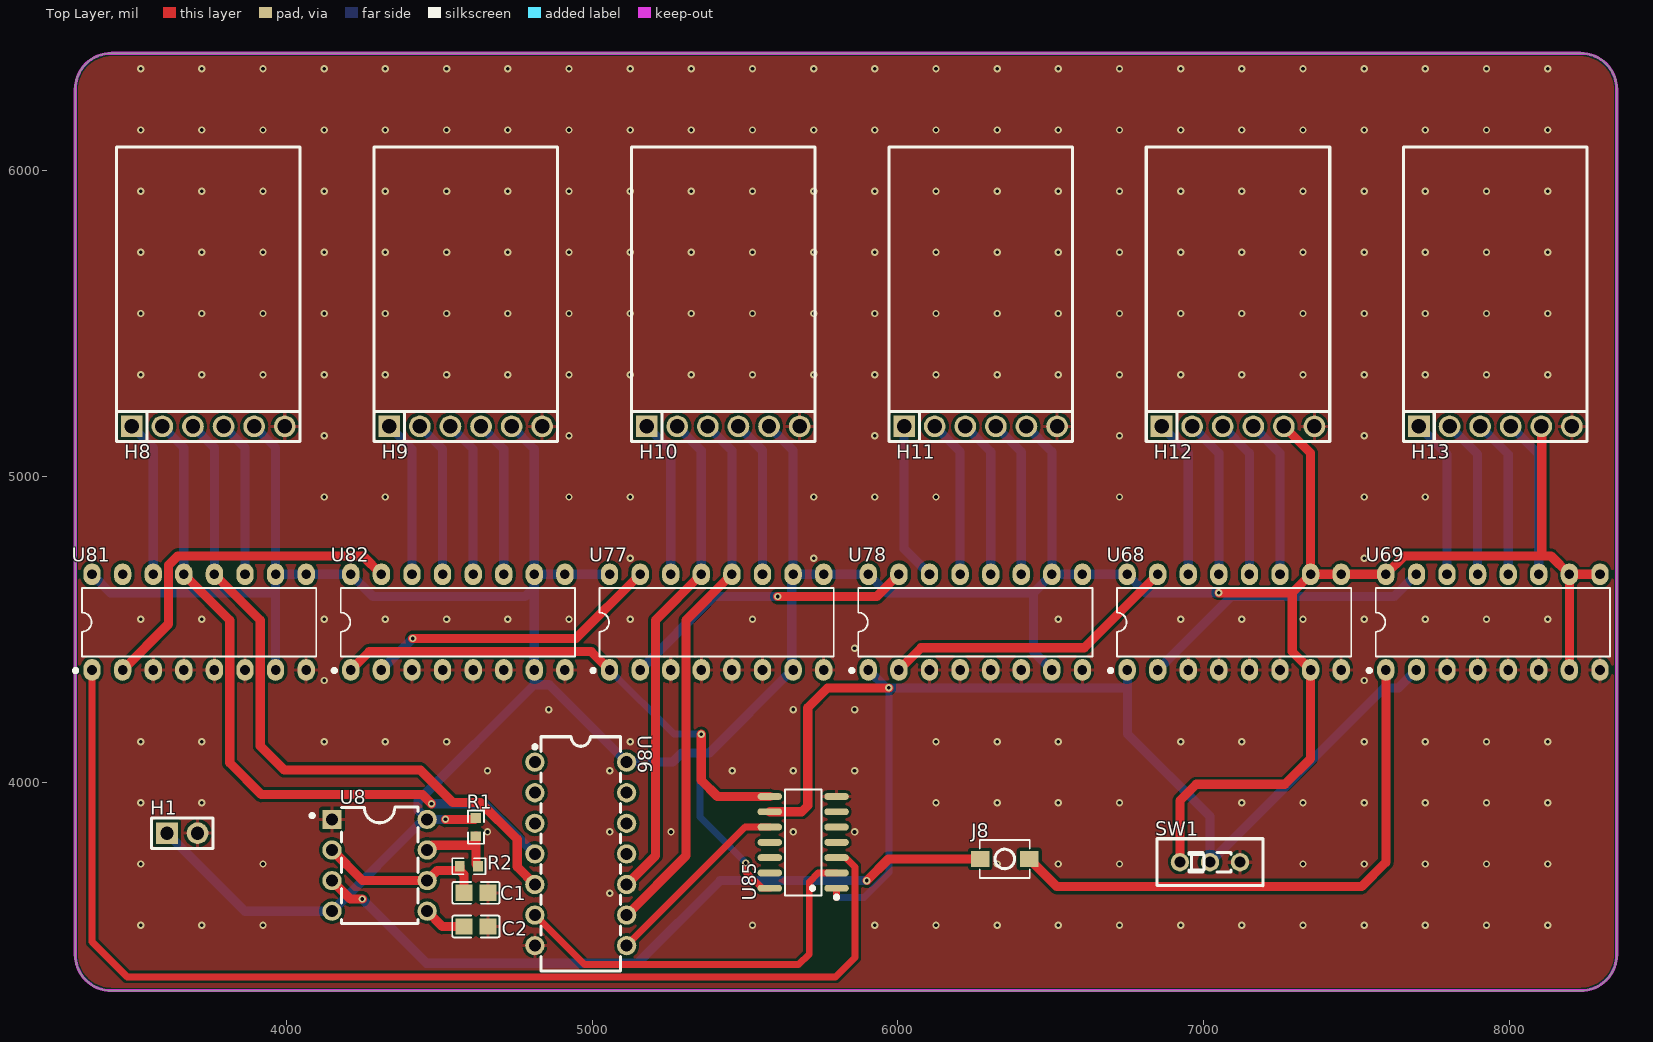
[diagram p0: Top Layer view]
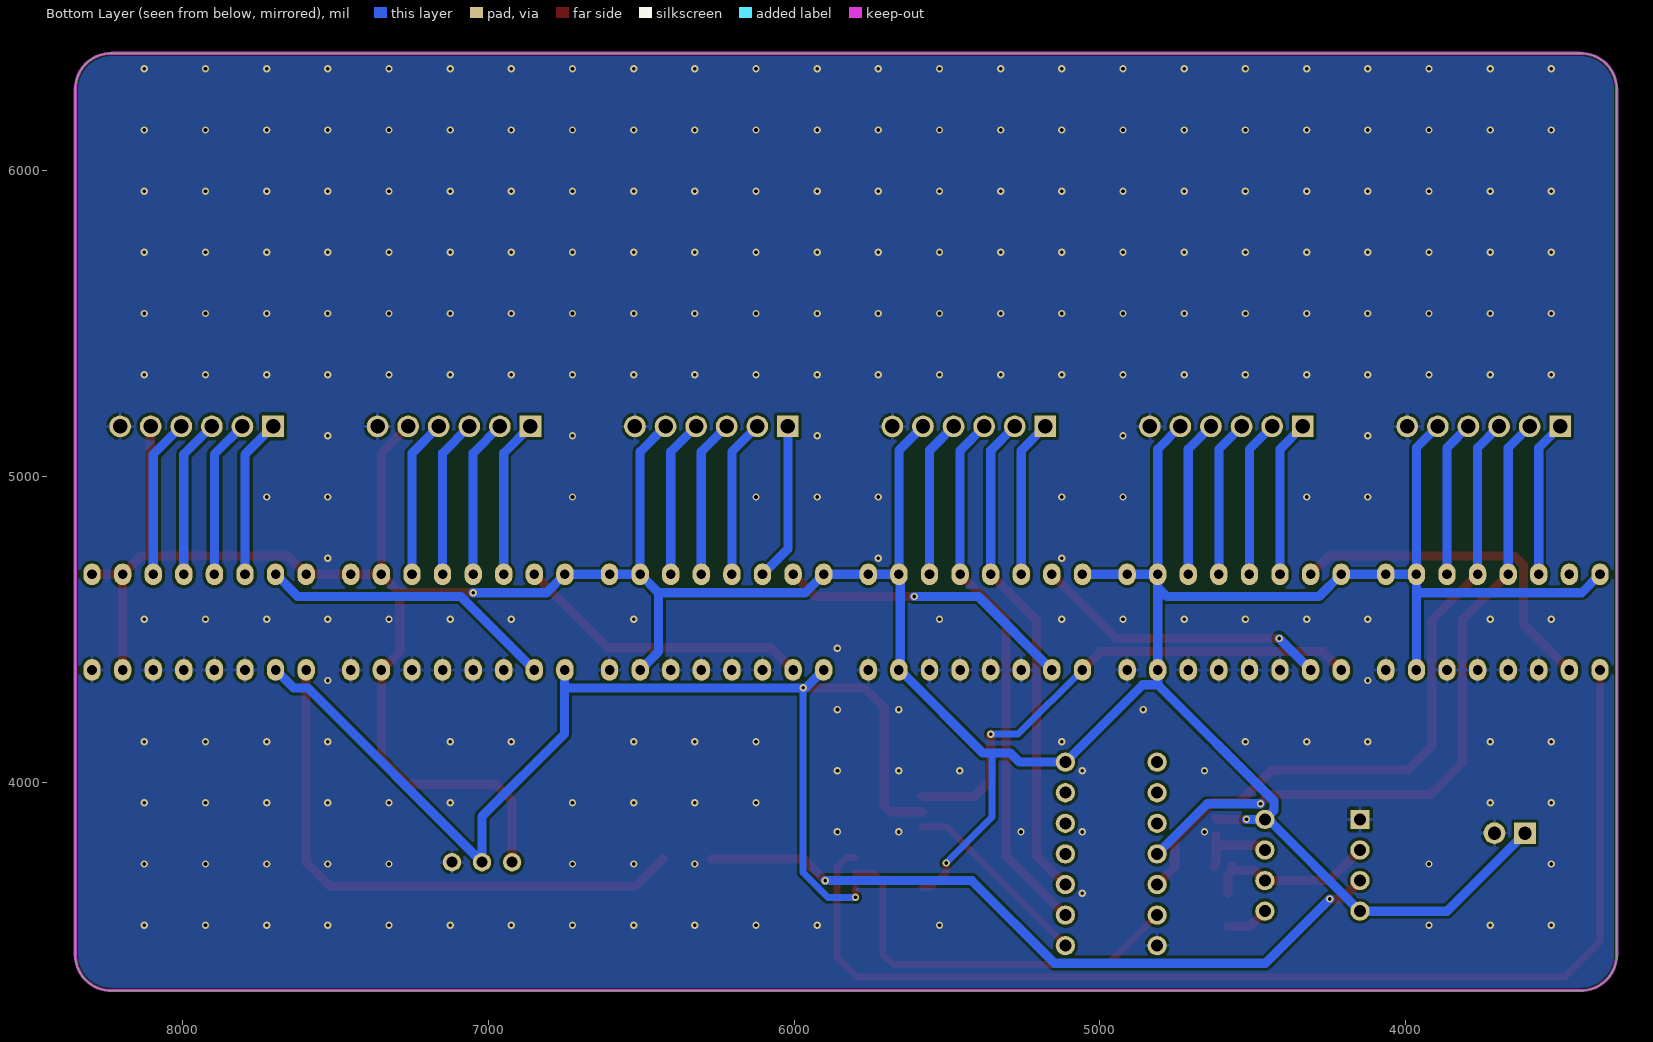
[diagram p1: Bottom Layer view, seen from below]
# Altium PCB MISC51760.pcbdoc
Units mil, origin at the board's own origin, x right, y up, seen from the top; angles counter-clockwise.
Board outline 5040 x 3065 mil, 2 copper layers (Top Layer, Bottom Layer), stack 62.206 mil thick; 22 components, 41 nets, 183 pads, 260 vias.

## Layer stack, top to bottom
Top Solder Mask Layer: solder mask 0.394, Dk 3.3
Top Layer: signal copper 1.379
Dielectric1: surface 59.449, FR4, Dk 4.5
Bottom Layer: signal copper 1.378
Bottom Solder Mask Layer: solder mask 0.394, Dk 3.3

## Board outline
3428.11,6385 ccw(c3428.11,6266.89) 3310,6266.89 3310,3438.11 ccw(c3428.11,3438.11) 3428.11,3320 8231.89,3320 ccw(c8231.89,3438.11) 8350,3438.11 8350,6266.89 ccw(c8231.89,6266.89) 8231.89,6385

## Design rules (kind name [scope] priority, off if disabled: settings)
BoardOutlineClearance copperThickness2oz_1 [All] p2 off: genericclearance=7.99 ignorepadtopadclearanceinfootprint=FALSE except(0: Arc-SplitContinuation Track-SplitContinuation SMDPad-SplitContinuation THPad-SplitContinuation Via-SplitContinuation Fill-SplitContinuation Region-SplitContinuation Poly-SplitContinuation Text-SplitContinuation Hole-SplitContinuation; 5.98: Arc-CutoutEdge Track-CutoutEdge SMDPad-CutoutEdge THPad-CutoutEdge Via-CutoutEdge Text-CutoutEdge; 6.89: Hole-OutlineEdge Hole-CutoutEdge; 10: Poly-OutlineEdge Poly-CutoutEdge; 11.81: Arc-OutlineEdge Track-OutlineEdge SMDPad-OutlineEdge THPad-OutlineEdge Via-OutlineEdge Fill-OutlineEdge Region-OutlineEdge Text-OutlineEdge Fill-CutoutEdge Region-CutoutEdge)
BoardOutlineClearance Plane_innerPlane_1 [All] p4 off: genericclearance=4.02 ignorepadtopadclearanceinfootprint=FALSE except(0: Arc-SplitContinuation Track-SplitContinuation SMDPad-SplitContinuation THPad-SplitContinuation Via-SplitContinuation Fill-SplitContinuation Region-SplitContinuation Poly-SplitContinuation Text-SplitContinuation Hole-SplitContinuation; 5.98: Arc-CutoutEdge Track-CutoutEdge SMDPad-CutoutEdge THPad-CutoutEdge Via-CutoutEdge Text-CutoutEdge; 6.89: Hole-OutlineEdge Hole-CutoutEdge; 10: Poly-OutlineEdge Poly-CutoutEdge; 11.81: Arc-OutlineEdge Track-OutlineEdge SMDPad-OutlineEdge THPad-OutlineEdge Via-OutlineEdge Fill-OutlineEdge Region-OutlineEdge Text-OutlineEdge Fill-CutoutEdge Region-CutoutEdge)
BoardOutlineClearance Copper_copperRegion_1 [All] p6 off: genericclearance=4.02 ignorepadtopadclearanceinfootprint=FALSE except(0: Arc-SplitContinuation Track-SplitContinuation SMDPad-SplitContinuation THPad-SplitContinuation Via-SplitContinuation Fill-SplitContinuation Region-SplitContinuation Poly-SplitContinuation Text-SplitContinuation Hole-SplitContinuation; 5.98: Arc-CutoutEdge Track-CutoutEdge SMDPad-CutoutEdge THPad-CutoutEdge Via-CutoutEdge Text-CutoutEdge; 6.89: Hole-OutlineEdge Hole-CutoutEdge; 10: Poly-OutlineEdge Poly-CutoutEdge; 11.81: Arc-OutlineEdge Track-OutlineEdge SMDPad-OutlineEdge THPad-OutlineEdge Via-OutlineEdge Fill-OutlineEdge Region-OutlineEdge Text-OutlineEdge Fill-CutoutEdge Region-CutoutEdge)
BoardOutlineClearance copperThickness1oz_1 [All] p8: genericclearance=4.02 ignorepadtopadclearanceinfootprint=FALSE except(0: Arc-SplitContinuation Track-SplitContinuation SMDPad-SplitContinuation THPad-SplitContinuation Via-SplitContinuation Fill-SplitContinuation Region-SplitContinuation Poly-SplitContinuation Text-SplitContinuation Hole-SplitContinuation; 5.98: Arc-CutoutEdge Track-CutoutEdge SMDPad-CutoutEdge THPad-CutoutEdge Via-CutoutEdge Text-CutoutEdge; 6.89: Hole-OutlineEdge Hole-CutoutEdge; 10: Poly-OutlineEdge Poly-CutoutEdge; 11.81: Arc-OutlineEdge Track-OutlineEdge SMDPad-OutlineEdge THPad-OutlineEdge Via-OutlineEdge Fill-OutlineEdge Region-OutlineEdge Text-OutlineEdge Fill-CutoutEdge Region-CutoutEdge)
Clearance copperThickness2oz [All] p1 off: gap=7.99 ignorepadtopadclearanceinfootprint=FALSE except(5.98: SMDPad-Track SMDPad-SMDPad THPad-Track SMDPad-THPad THPad-THPad Track-Via SMDPad-Via THPad-Via Via-Via Fill-SMDPad Region-SMDPad Fill-THPad Region-THPad Fill-Via Region-Via Fill-Fill Fill-Region Region-Region Arc-Track Arc-SMDPad Arc-THPad Arc-Via Fill-Arc Region-Arc Arc-Arc Text-Track SMDPad-Text Text-THPad Text-Via Fill-Text Region-Text Arc-Text Text-Text; 6.89: Hole-Track Hole-SMDPad Hole-THPad Hole-Via Fill-Hole Region-Hole Hole-Arc Hole-Text; 10: Poly-Track Poly-SMDPad Poly-THPad Poly-Via Poly-Fill Poly-Region Poly-Poly Poly-Arc Poly-Text Poly-Hole; 11.81: Fill-Track Region-Track)
Clearance Plane_innerPlane [All] p3 off: gap=4.02 ignorepadtopadclearanceinfootprint=FALSE except(5.98: SMDPad-Track SMDPad-SMDPad THPad-Track SMDPad-THPad THPad-THPad Track-Via SMDPad-Via THPad-Via Via-Via Fill-SMDPad Region-SMDPad Fill-THPad Region-THPad Fill-Via Region-Via Fill-Fill Fill-Region Region-Region Arc-Track Arc-SMDPad Arc-THPad Arc-Via Fill-Arc Region-Arc Arc-Arc Text-Track SMDPad-Text Text-THPad Text-Via Fill-Text Region-Text Arc-Text Text-Text; 6.89: Hole-Track Hole-SMDPad Hole-THPad Hole-Via Fill-Hole Region-Hole Hole-Arc Hole-Text; 10: Poly-Track Poly-SMDPad Poly-THPad Poly-Via Poly-Fill Poly-Region Poly-Poly Poly-Arc Poly-Text Poly-Hole; 11.81: Fill-Track Region-Track)
Clearance Copper_copperRegion [All] p5 off: gap=4.02 ignorepadtopadclearanceinfootprint=FALSE except(5.98: SMDPad-Track SMDPad-SMDPad THPad-Track SMDPad-THPad THPad-THPad Track-Via SMDPad-Via THPad-Via Via-Via Fill-SMDPad Region-SMDPad Fill-THPad Region-THPad Fill-Via Region-Via Fill-Fill Fill-Region Region-Region Arc-Track Arc-SMDPad Arc-THPad Arc-Via Fill-Arc Region-Arc Arc-Arc Text-Track SMDPad-Text Text-THPad Text-Via Fill-Text Region-Text Arc-Text Text-Text; 6.89: Hole-Track Hole-SMDPad Hole-THPad Hole-Via Fill-Hole Region-Hole Hole-Arc Hole-Text; 10: Poly-Track Poly-SMDPad Poly-THPad Poly-Via Poly-Fill Poly-Region Poly-Poly Poly-Arc Poly-Text Poly-Hole; 11.81: Fill-Track Region-Track)
Clearance copperThickness1oz [All] p7: gap=4.02 ignorepadtopadclearanceinfootprint=FALSE except(5.98: SMDPad-Track SMDPad-SMDPad THPad-Track SMDPad-THPad THPad-THPad Track-Via SMDPad-Via THPad-Via Via-Via Fill-SMDPad Region-SMDPad Fill-THPad Region-THPad Fill-Via Region-Via Fill-Fill Fill-Region Region-Region Arc-Track Arc-SMDPad Arc-THPad Arc-Via Fill-Arc Region-Arc Arc-Arc Text-Track SMDPad-Text Text-THPad Text-Via Fill-Text Region-Text Arc-Text Text-Text; 6.89: Hole-Track Hole-SMDPad Hole-THPad Hole-Via Fill-Hole Region-Hole Hole-Arc Hole-Text; 10: Poly-Track Poly-SMDPad Poly-THPad Poly-Via Poly-Fill Poly-Region Poly-Poly Poly-Arc Poly-Text Poly-Hole; 11.81: Fill-Track Region-Track)
DiffPairsRouting differentialPair [All] p1: maxlimit=6 minlimit=6 mostfreqgap=6 toplayer_minwidth=5 toplayer_prefwidth=10 toplayer_maxwidth=100 toplayer_mingap=6 toplayer_prefgap=6 toplayer_maxgap=6 bottomlayer_minwidth=5 bottomlayer_prefwidth=10 bottomlayer_maxwidth=100 bottomlayer_mingap=6 bottomlayer_prefgap=6 bottomlayer_maxgap=6 maxuncoupledlength=10
HoleToHoleClearance otherClearance [All] p1: gap=11.81 allowstackedmicrovias=TRUE
Length netLength [All] p1: minlimit=0 maxlimit=0
PasteMaskExpansion pasteMaskExpansion [All] p1: expansion=0
PlaneConnect innerPlane [All] p1: planeconnectstyle=Relief reliefexpansion=20 reliefentries=4 reliefconductorwidth=10 reliefairgap=10
PolygonConnect copperRegion [All] p1: connectstyle=Relief reliefconductorwidth=10 reliefentries=4 polygonreliefangle="90 Angle" airgapwidth=10 via.connectstyle=Relief via.reliefconductorwidth=10 via.reliefentries=4 via.polygonreliefangle="90 Angle" via.airgapwidth=10
RoutingVias viaSize [All] p1: holewidth=12.01 width=24.02 viastyle="Through Hole" minholewidth=11.81 minwidth=19.68 maxholewidth=248.03 maxwidth=393.7
SolderMaskExpansion solderMaskExpansion [IsVia] p1: expansion=-1000 istentingtop=TRUE
SolderMaskExpansion solderMaskExpansion [All] p2: expansion=2.01 istentingtop=FALSE
Width copperThickness2oz_2 [All] p1 off: maxlimit=100 minlimit=8 preferedwidth=10
Width copperThickness1oz_2 [All] p2: maxlimit=100 minlimit=5 preferedwidth=30

## Components (designator, comment, footprint, x,y, rotation, side; value= is the part's Value field where it differs from the comment)
C1 "1uF" C0805 4620,3640 r180 top
C2 "10nF" C0805 4620,3530 r180 top
H1 "" HDR-TH_2P-P2.54-V-M-1 3660,3835 r0 top
H8 "" HDR-TH_6P-P2.54-V-M-1 3745,5165 r0 top
H9 "" HDR-TH_6P-P2.54-V-M-1 4586.66,5165 r0 top
H10 "" HDR-TH_6P-P2.54-V-M-1 5428.33,5165 r0 top
H11 "" HDR-TH_6P-P2.54-V-M-1 6269.99,5165 r0 top
H12 "" HDR-TH_6P-P2.54-V-M-1 7111.65,5165 r0 top
H13 "" HDR-TH_6P-P2.54-V-M-1 7953.31,5165 r0 top
J8 "轻触按键3*4*H" SW-SMD_L4.0-W2.9-LS5.0 6349.05,3750.66 r0 top
R1 "10k" R0603 4620,3855 r90 top
R2 "2.2k" R0603 4597.22,3726.91 r0 top
SW1 "开关" SW-TH_SS-12D01-GX 7020,3740 r0 top
U8 "NE555PE4" PDIP-8_L9.6-W6.4-P2.54-LS7.9-BL-1 4305,3730 r270 top
U68 "74LS160D" PDIP-16_L19.3-W6.4-P2.54-LS7.94-BL 7099,4525 r0 top
U69 "74LS160D" PDIP-16_L19.3-W6.4-P2.54-LS7.94-BL 7945,4525 r0 top
U77 "74LS160D" PDIP-16_L19.3-W6.4-P2.54-LS7.94-BL 5407,4525 r0 top
U78 "74LS160D" PDIP-16_L19.3-W6.4-P2.54-LS7.94-BL 6253,4525 r0 top
U81 "74LS160D" PDIP-16_L19.3-W6.4-P2.54-LS7.94-BL 3715,4525 r0 top
U82 "74LS160D" PDIP-16_L19.3-W6.4-P2.54-LS7.94-BL 4561,4525 r0 top
U85 "SN74LS08DR(LX)" SOIC-14_L8.7-W3.9-P1.27-LS6.0-BL 5690,3805 r90 top
U86 "SN74LS00N(LX)" PDIP-14_L19.3-W6.4-P2.54-LS7.9-BL 4962.75,3767.25 r270 top

## Footprints (in the part's own frame and the unit in brackets; to place one, negate y for a bottom-side part, rotate by r counter-clockwise, add the part's x,y. Pads: shape width x height; smd on the part's side, far side on the other; paste and mask are expansions set on the pad)
C0805 [mm]
  rect 1.41x1.35 smd paste-100 mask+0.051: 1(-1,0) 2(1,0)
  silkscreen extent -1.96,-0.9 1.96,0.9
HDR-TH_2P-P2.54-V-M-1 [mm]
  rect 1.8x1.8 hole 1.1: 1(-1.27,0)
  round 1.8 hole 1.1: 2(1.27,0)
  silkscreen extent -2.54,-1.27 2.54,1.27
HDR-TH_6P-P2.54-V-M-1 [mm]
  rect 1.8x1.8 hole 1.2: 1(-6.35,0)
  round 1.8 hole 1.2: 2(-3.81,0) 3(-1.27,0) 4(1.27,0) 5(3.81,0) 6(6.35,0)
  silkscreen extent -7.62,-1.25 7.62,23.2
PDIP-8_L9.6-W6.4-P2.54-LS7.9-BL-1 [mil]
  rect 63x63 hole 39.37: 1(-150,-155.51)
  round 63 hole 39.37: 2(-50,-155.51) 3(50,-155.51) 4(150,-155.51) 5(150,155.52) 6(50,155.52) 7(-50,155.52) 8(-150,155.52)
  silkscreen extent -190,-226 190,125
PDIP-14_L19.3-W6.4-P2.54-LS7.9-BL [mm]
  round 1.6 hole 1: 1(-7.62,-3.81) 2(-5.08,-3.81) 3(-2.54,-3.81) 4(0,-3.81) 5(2.54,-3.81) 6(5.08,-3.81) 7(7.62,-3.81) 8(7.62,3.81) 9(5.08,3.81) 10(2.54,3.81) 11(0,3.81) 12(-2.54,3.81) 13(-5.08,3.81) 14(-7.62,3.81)
  silkscreen extent -9.73,-3.96 9.73,3.3
PDIP-16_L19.3-W6.4-P2.54-LS7.94-BL [mm]
  oval 1.44x1.8 hole 0.8: 1(-8.89,-3.97) 2(-6.35,-3.97) 3(-3.81,-3.97) 4(-1.27,-3.97) 5(1.27,-3.97) 6(3.81,-3.97) 7(6.35,-3.97) 8(8.89,-3.97) 9(8.89,3.97) 10(6.35,3.97) 11(3.81,3.97) 12(1.27,3.97) 13(-1.27,3.97) 14(-3.81,3.97) 15(-6.35,3.97) 16(-8.89,3.97)
  silkscreen extent -10.41,-4.17 9.73,2.84
R0603 [mil]
  rect 31.75x34.02 smd paste-3937.01 mask+2: 1(-29.66,0) 2(29.66,0)
  silkscreen extent -55,-26 55,26
SOIC-14_L8.7-W3.9-P1.27-LS6.0-BL [mil]
  oval 22.6x80.24 smd: 1(-150,-109.02) 2(-100,-109.02) 3(-50,-109.02) 4(0,-109.02) 5(50,-109.02) 6(100,-109.02) 7(150,-109.02) 8(150,109.02) 9(100,109.02) 10(50,109.02) 11(0,109.02) 12(-50,109.02) 13(-100,109.02) 14(-150,109.02)
  silkscreen extent -185,-115 173,60
SW-SMD_L4.0-W2.9-LS5.0 [mm]
  rect 1.53x1.36 smd: 1(-2.035,0) 2(2.035,0)
  silkscreen extent -2.08,-1.58 2.08,1.58
SW-TH_SS-12D01-GX [mil]
  round 60 hole 36: 1(-98.43,0) 2(-0.01,0) 3(98.42,0)
  silkscreen extent -173,-77 173,77

## Via types
v1: diameter 24.02, hole 12, Top Layer to Bottom Layer, 260 vias

## Nets (pads, with @x,y where several pads share a name; then routed paths per layer and width w, separated by ;. In a path a pad name is that pad's centre, name@x,y a point inside that pad or via, vN(x,y) a via of type N, cw(c..) or ccw(c..) an arc to the next point about the centre after c; other vN are vias at no path point)
$1N38628: H12.1 U68.14 | length 519.9
  Bottom Layer w30: H12.1 6949,5077.65 U68.14
$1N38636: H12.2 U68.13 | length 519.9
  Bottom Layer w30: H12.2 7049,5077.65 U68.13
$1N38644: H12.3 U68.12 | length 519.9
  Bottom Layer w30: H12.3 7149,5077.65 U68.12
$1N38648: H12.4 U68.11 | length 519.9
  Bottom Layer w30: H12.4 7249,5077.65 U68.11
$1N39456: H13.1 U69.14 | length 521.7
  Bottom Layer w30: H13.1 7795,5073.31 U69.14
$1N39460: H13.2 U69.13 | length 521.7
  Bottom Layer w30: H13.2 7895,5073.31 U69.13
$1N39464: H13.3 U69.12 | length 521.7
  Bottom Layer w30: H13.3 7995,5073.31 U69.12
$1N39468: H13.4 U69.11 | length 521.7
  Bottom Layer w30: H13.4 8095,5073.31 U69.11
$1N39487: U68.2 U69.15 | length 975.5
  Bottom Layer w30: U68.2 7089,4608.7 7622.4,4608.7 U69.15
$1N58076: R1.1 R2.2 U8.7 | length 267.1
  Top Layer w30: U8.7 4475.85,3795.34 4620,3795.34 ; R1.1 4620,3795.34 ; R2.2 4620,3733.8 4620,3795.34
$1N58077: C1.2 R2.1 U8.2 U8.6 | length 565.5
  Top Layer w30: U8.2 4249.49,3680 U8.6 4493.58,3713.07 R2.1@4567.56,3713.07 ; R2.1 R2.1@4567.56,3713.07 ; C1.2 4580.63,3700 R2.1@4567.56,3713.07
$1N58078: C2.2 U8.5 | length 140.8
  Top Layer w30: U8.5 4510.51,3530 C2.2
$1N58085: J8.1 U8.3 | length 2372.4
  Top Layer w30: U8.3 4209.49,3620 v1(4248.28,3620) ; v1(5898.28,3680) 5968.93,3750.66 J8.1
  Bottom Layer w30: v1(4248.28,3620) 4458.28,3410 5148.28,3410 5418.28,3680 v1(5898.28,3680)
$1N59924: H11.4 U78.11 | length 518.1
  Bottom Layer w30: H11.4 6403,5081.99 U78.11
$1N59928: H11.3 U78.12 | length 518.1
  Bottom Layer w30: H11.3 6303,5081.99 U78.12
$1N59932: H11.1 U78.14 | length 518.1
  Bottom Layer w30: H11.1 6019.99,4764.31 U78.14
$1N59936: H11.2 U78.13 | length 518.1
  Bottom Layer w30: H11.2 6203,5081.99 U78.13
$1N59943: U77.2 U78.15 | length 975.5
  Top Layer w30: v1(5607,4608.7) 5930.4,4608.7 U78.15
  Bottom Layer w30: U77.2 5397,4608.7 v1(5607,4608.7)
$1N59947: H10.3 U77.12 U86.9 | length 1772.9
  Top Layer w30: U86.9 5307,3761.49 5307,4531.3 U77.12
  Bottom Layer w30: H10.3 5457,5086.33 U77.12
$1N59951: H10.2 U77.13 U86.10 | length 1631.5
  Top Layer w30: U86.10 5207,3761.49 5207,4531.3 U77.13
  Bottom Layer w30: H10.2 5357,5086.33 U77.13
$1N59955: H10.1 U77.14 | length 516.3
  Bottom Layer w30: H10.1 5257,5086.33 U77.14
$1N59959: H10.4 U77.11 | length 516.3
  Bottom Layer w30: H10.4 5557,5086.33 U77.11
$1N60960: H9.4 U82.11 | length 514.5
  Bottom Layer w30: H9.4 4711,5090.66 U82.11
$1N60964: H9.3 U82.12 | length 514.5
  Bottom Layer w30: H9.3 4611,5090.66 U82.12
$1N60968: H9.1 U82.14 | length 514.5
  Bottom Layer w30: H9.1 4411,5090.66 U82.14
$1N60972: H9.2 U82.13 | length 514.5
  Bottom Layer w30: H9.2 4511,5090.66 U82.13
$1N60979: U81.2 U82.15 | length 1138
  Top Layer w30: U81.2 3615,4518.7 3615,4711.3 3645,4741.3 4251,4741.3 U82.15
$1N60983: H8.3 U81.12 U86.5 | length 2274.1
  Top Layer w30: U81.12 3915,4531.3 3915,4120 3993.35,4041.65 4438.35,4041.65 4545,3935 4635,3935 4755,3815 4755,3725 U86.5
  Bottom Layer w30: H8.3 3765,5095 U81.12
$1N60987: H8.2 U81.13 U86.4 | length 2312.2
  Top Layer w30: U81.13 3815,4531.3 3815,4065 3918.7,3961.3 4445,3961.3 v1(4475,3931.3)
  Bottom Layer w30: H8.2 3665,5095 U81.13 ; v1(4475,3931.3) 4648.7,3931.3 U86.4
$1N60991: H8.1 U81.14 | length 512.7
  Bottom Layer w30: H8.1 3565,5095 U81.14
$1N60995: H8.4 U81.11 | length 512.7
  Bottom Layer w30: H8.4 3865,5095 U81.11
$1N65984: J8.2 U69.1 | length 1864.7
  Top Layer w30: J8.2 6519.17,3660.66 7515.66,3660.66 7595,3740 U69.1
$1N66441: U85.2 U86.6 | length 1316
  Top Layer w22.6: U86.6 4975,3405 5675,3405 5709.98,3439.98 5709.98,3675.96 5739.02,3705 U85.2
$1N66464: U81.1 U85.3 | length 3825.3
  Top Layer w22.6: U81.1 3365,3480 3480,3365 5795,3365 5859.02,3429.02 5859.02,3725 5829.02,3755 U85.3
$1N66546: U77.15 U82.2 | length 975.5
  Top Layer w30: v1(4413.6,4471.3) 4947,4471.3 U77.15
  Bottom Layer w30: U82.2 v1(4413.6,4471.3)
$1N66559: U68.15 U78.2 | length 975.5
  Top Layer w30: U78.2 6075.6,4441.3 6609,4441.3 U68.15
$1N66593: U85.10 U86.8 | length 628.8
  Top Layer w22.6: U86.8 5500.51,3855 U85.10
$1N66598: U77.1 U82.1 U85.8 | length 1679.3
  Top Layer w30: U82.1 4271,4428.7 4997,4428.7 U77.1 ; v1(5357,4158.7) 5357,4008 5410,3955 U85.8
  Bottom Layer w22.6: U77.1 5267,4158.7 v1(5357,4158.7)
$1N66613: SW1.2 U68.1 U69.2 U78.1 U85.1 U85.9 | length 4130.4
  Top Layer w22.6: v1(5799.02,3625) U85.1
  Top Layer w30: U85.9 5685,3905 5705,3925 5705,4245 5770,4310 v1(5969.99,4310)
  Bottom Layer w22.6: v1(5799.02,3625) 5889.02,3625 5969.99,3705.97 v1(5969.99,4310)
  Bottom Layer w30: U78.1 5961.7,4310 v1(5969.99,4310) 6749.99,4310 ; U68.1 6749.99,4367.7 6749.99,4310 ; U69.2 7636.3,4310 7589.99,4310 SW1.2 7019.99,3890 6749.99,4160 6749.99,4310
GND: C1.1 C2.1 H1.2 H8.6 H9.6 H10.6 H11.6 H12.6 H13.6 SW1.3 U8.1 U68.3 U68.4 U68.5 U68.6 U68.8 U69.3 U69.4 U69.5 U69.6 U69.8 U77.3 U77.4 U77.5 U77.6 U77.8 U78.3 U78.4 U78.5 U78.6 U78.8 U81.3 U81.4 U81.5 U81.6 U81.8 U82.3 U82.4 U82.5 U82.6 U82.8 U85.7 U86.7
  other v1: 3524.1,3534.1 3724.1,3534.1 3924.1,3534.1 5524.1,3534.1 5924.1,3534.1 6124.1,3534.1 6324.1,3534.1 6524.1,3534.1 6724.1,3534.1 6924.1,3534.1 7124.1,3534.1 7324.1,3534.1 7524.1,3534.1 7724.1,3534.1 7924.1,3534.1 8124.1,3534.1 5058.05,3639.1 3524.1,3734.1 3924.1,3734.1 6324.1,3734.1 6524.1,3734.1 6724.1,3734.1 7324.1,3734.1 7524.1,3734.1 7724.1,3734.1 7924.1,3734.1 8124.1,3734.1 4658.05,3839.1 5058.05,3839.1 5258.05,3839.1 5658.05,3839.1 5858.05,3839.1 3524.1,3934.1 3724.1,3934.1 6124.1,3934.1 6324.1,3934.1 6524.1,3934.1 6724.1,3934.1 7124.1,3934.1 7324.1,3934.1 7524.1,3934.1 7724.1,3934.1 7924.1,3934.1 8124.1,3934.1 4658.05,4039.1 5058.05,4039.1 5458.05,4039.1 5658.05,4039.1 5858.05,4039.1 3524.1,4134.1 3724.1,4134.1 4124.1,4134.1 4324.1,4134.1 4524.1,4134.1 5124.1,4134.1 6124.1,4134.1 6324.1,4134.1 6524.1,4134.1 6924.1,4134.1 7124.1,4134.1 7524.1,4134.1 7724.1,4134.1 7924.1,4134.1 8124.1,4134.1 4858.05,4239.1 5658.05,4239.1 5858.05,4239.1 4124.1,4334.1 7524.1,4334.1 5858.05,4439.1 3524.1,4534.1 3724.1,4534.1 4124.1,4534.1 4324.1,4534.1 4524.1,4534.1 4724.1,4534.1 4924.1,4534.1 5124.1,4534.1 5524.1,4534.1 6524.1,4534.1 6924.1,4534.1 7124.1,4534.1 7324.1,4534.1 7524.1,4534.1 7724.1,4534.1 7924.1,4534.1 8124.1,4534.1 5124.1,4734.1 5724.1,4734.1 7524.1,4734.1 4124.1,4934.1 4324.1,4934.1 4924.1,4934.1 5124.1,4934.1 5724.1,4934.1 5924.1,4934.1 6124.1,4934.1 6724.1,4934.1 7524.1,4934.1 7724.1,4934.1 4124.1,5134.1 4924.1,5134.1 5924.1,5134.1 6724.1,5134.1 7524.1,5134.1 3524.1,5334.1 3724.1,5334.1 3924.1,5334.1 4124.1,5334.1 4324.1,5334.1 4524.1,5334.1 4724.1,5334.1 4924.1,5334.1 5124.1,5334.1 5324.1,5334.1 5524.1,5334.1 5724.1,5334.1 5924.1,5334.1 6124.1,5334.1 6324.1,5334.1 6524.1,5334.1 6724.1,5334.1 6924.1,5334.1 7124.1,5334.1 7324.1,5334.1 7524.1,5334.1 7724.1,5334.1 7924.1,5334.1 8124.1,5334.1 3524.1,5534.1 3724.1,5534.1 3924.1,5534.1 4124.1,5534.1 4324.1,5534.1 4524.1,5534.1 4724.1,5534.1 4924.1,5534.1 5124.1,5534.1 5324.1,5534.1 5524.1,5534.1 5724.1,5534.1 5924.1,5534.1 6124.1,5534.1 6324.1,5534.1 6524.1,5534.1 6724.1,5534.1 6924.1,5534.1 7124.1,5534.1 7324.1,5534.1 7524.1,5534.1 7724.1,5534.1 7924.1,5534.1 8124.1,5534.1 3524.1,5734.1 3724.1,5734.1 3924.1,5734.1 4124.1,5734.1 4324.1,5734.1 4524.1,5734.1 4724.1,5734.1 4924.1,5734.1 5124.1,5734.1 5324.1,5734.1 5524.1,5734.1 5724.1,5734.1 5924.1,5734.1 6124.1,5734.1 6324.1,5734.1 6524.1,5734.1 6724.1,5734.1 6924.1,5734.1 7124.1,5734.1 7324.1,5734.1 7524.1,5734.1 7724.1,5734.1 7924.1,5734.1 8124.1,5734.1 3524.1,5934.1 3724.1,5934.1 3924.1,5934.1 4124.1,5934.1 4324.1,5934.1 4524.1,5934.1 4724.1,5934.1 4924.1,5934.1 5124.1,5934.1 5324.1,5934.1 5524.1,5934.1 5724.1,5934.1 5924.1,5934.1 6124.1,5934.1 6324.1,5934.1 6524.1,5934.1 6724.1,5934.1 6924.1,5934.1 7124.1,5934.1 7324.1,5934.1 7524.1,5934.1 7724.1,5934.1 7924.1,5934.1 8124.1,5934.1 3524.1,6134.1 3724.1,6134.1 3924.1,6134.1 4124.1,6134.1 4324.1,6134.1 4524.1,6134.1 4724.1,6134.1 4924.1,6134.1 5124.1,6134.1 5324.1,6134.1 5524.1,6134.1 5724.1,6134.1 5924.1,6134.1 6124.1,6134.1 6324.1,6134.1 6524.1,6134.1 6724.1,6134.1 6924.1,6134.1 7124.1,6134.1 7324.1,6134.1 7524.1,6134.1 7724.1,6134.1 7924.1,6134.1 8124.1,6134.1 3524.1,6334.1 3724.1,6334.1 3924.1,6334.1 4124.1,6334.1 4324.1,6334.1 4524.1,6334.1 4724.1,6334.1 4924.1,6334.1 5124.1,6334.1 5324.1,6334.1 5524.1,6334.1 5724.1,6334.1 5924.1,6334.1 6124.1,6334.1 6324.1,6334.1 6524.1,6334.1 6724.1,6334.1 6924.1,6334.1 7124.1,6334.1 7324.1,6334.1 7524.1,6334.1 7724.1,6334.1 7924.1,6334.1 8124.1,6334.1
VCC: H1.1 H8.5 H9.5 H10.5 H11.5 H12.5 H13.5 R1.2 SW1.1 U8.4 U8.8 U68.7 U68.9 U68.10 U68.16 U69.7 U69.9 U69.10 U69.16 U77.7 U77.9 U77.10 U77.16 U78.7 U78.9 U78.10 U78.16 U81.7 U81.9 U81.10 U81.16 U82.7 U82.9 U82.10 U82.16 U85.14 U86.14 | length 13864.2
  Top Layer w22.6: v1(5502.75,3737.25) 5502.75,3707.25 5555,3655 U85.14
  Top Layer w30: v1(4520.51,3880) 4615.34,3880 R1.2 ; SW1.1 6921.57,3941.28 6975.04,3994.74 7264.74,3994.74 7349,4079 U68.7 7289,4428.7 7289,4621.3 ; v1(7049,4621.3) 7289,4621.3 ; H12.5 7349,5077.65 U68.10 ; H13.5 8105,5163.31 8105,4741.3 ; U69.7 U69.10 ; U69.9 U69.10 ; 7289,4621.3 U68.10 ; U68.10 U68.9 U69.16 7655,4741.3 8105,4741.3 ; 8105,4741.3 8135,4741.3 U69.10
  Bottom Layer w22.6: 5352.75,4097.25 5352.75,3887.25 v1(5502.75,3737.25)
  Bottom Layer w30: U81.16 3425,4621.3 3965,4621.3 ; H1.1 3865,3580 U8.4 4449.49,3880 U8.8 ; H8.5 3965,5095 U81.10 ; U81.7 3965,4621.3 ; v1(4520.51,3880) U8.8 ; H9.5 4811,5090.66 U82.10 ; U77.16 U82.9 U82.10 ; H10.5 5657,5086.33 U77.10 ; U77.7 U77.7@5652.75,4367.25 ; H11.5 6503,5081.99 U78.10 ; U78.7 6443,4428.7 6443,4621.3 ; v1(7049,4621.3) 6809,4621.3 U68.16 U78.9 U78.10 ; 3965,4621.3 U81.10 ; U81.10 U81.9 U82.16 4283.6,4608.7 4781,4608.7 4811,4638.7 ; U8.8 4430.51,3910 4430.51,3940 4811,4320.49 ; 4811,4320.49 U82.7 4811,4638.7 ; 4811,4320.49 4859.51,4320.49 U86.14 5262.75,4067.25 5292.75,4097.25 5352.75,4097.25 5382.75,4097.25 U77.7@5652.75,4367.25 ; 4811,4638.7 U82.10 ; U77.7@5652.75,4367.25 5652.75,4677.05 U77.10 ; U77.10 U77.9 U78.16 5963,4621.3 6443,4621.3 ; 6443,4621.3 U78.10
pads on no net: U81.15 U85.4 U85.5 U85.6 U85.11 U85.12 U85.13 U86.1 U86.2 U86.3 U86.11 U86.12 U86.13

## Polygon pours and split planes (outlines as drawn)
GND on Top Layer (solid, remove dead copper, pour order 0): 3205,6505 3205,3100 8740,3100 8740,6505
GND on Bottom Layer (solid, remove dead copper, pour order 2): 3000,6555 3000,3000 8940,3000 8940,6555

## Keep-outs
Board Outline Layer:
  the board outline again, w10